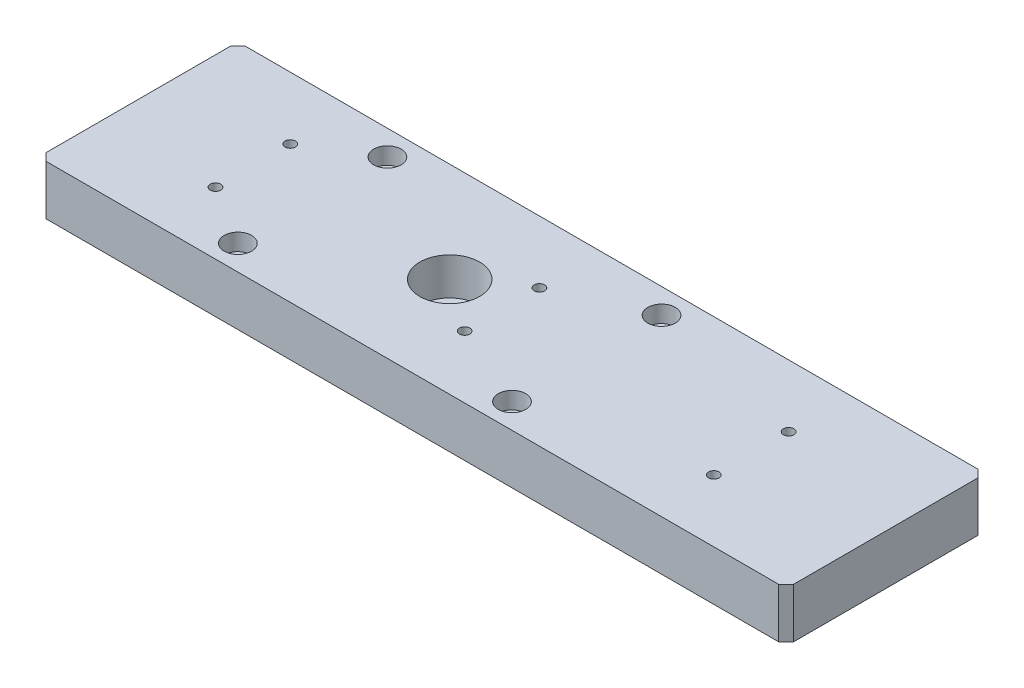
from build123d import *

# Parameters (mm, degrees)
SKETCH_1_W                = 300
SKETCH_1_H                = 80
EXTRUDE_1_DEPTH           = 20
CHAMFER_1_SIZE            = 3
HOLE_WIZARD_1_D           = 15.5
HOLE_WIZARD_1_DEPTH       = 25
HOLE_WIZARD_1_CBORE_D     = 24
HOLE_WIZARD_1_CBORE_DEPTH = 15
HOLE_WIZARD_1_TIP         = 4.656669797
HOLE_WIZARD_0_D           = 6.6
HOLE_WIZARD_0_DEPTH       = 25
HOLE_WIZARD_0_CBORE_D     = 11
HOLE_WIZARD_0_CBORE_DEPTH = 6.8
HOLE_WIZARD_0_TIP         = 1.982840043
SKETCH_6_R                = 10
SKETCH_6_R_2              = 8.1
CUT_EXTRUDE_1_DEPTH       = 2
HOLE_WIZARD_M5_1_D        = 4.2
HOLE_WIZARD_M5_2_D        = 4.2
HOLE_WIZARD_M5_2_DEPTH    = 12.4
HOLE_WIZARD_M5_2_TIP      = 1.2618073


with BuildPart() as part:
    # 草图1 → 凸台-拉伸1 (new body)
    with BuildSketch(Plane(origin=(0, 0, 0), x_dir=(1, 0, 0), z_dir=(0, 1, 0))):
        Rectangle(SKETCH_1_W, SKETCH_1_H)
    extrude(amount=EXTRUDE_1_DEPTH)

    # 倒角1
    chamfer_1_edges = [part.edges().sort_by_distance(p)[0] for p in [
        (150, 10, 40),
        (-150, 10, 40),
        (-150, 10, -40),
        (150, 10, -40),
    ]]
    chamfer(chamfer_1_edges, length=CHAMFER_1_SIZE)

    # 打孔尺寸(%根据)内六角圆柱头螺钉的类型1
    with Locations(Plane(origin=(0, 20, 0), x_dir=(1, 0, 0), z_dir=(0, 1, 0))):
        with Locations((-25, 0)):
            CounterBoreHole(HOLE_WIZARD_1_D / 2, HOLE_WIZARD_1_CBORE_D / 2, HOLE_WIZARD_1_CBORE_DEPTH, depth=HOLE_WIZARD_1_DEPTH)
            with Locations((0, 0, -(HOLE_WIZARD_1_DEPTH + HOLE_WIZARD_1_TIP / 2))):  # 118° drill point
                Cone(0, HOLE_WIZARD_1_D / 2, HOLE_WIZARD_1_TIP, mode=Mode.SUBTRACT)

    # 打孔尺寸(%根据)内六角圆柱头螺钉的类型0
    with Locations(Plane(origin=(0, 20, 0), x_dir=(1, 0, 0), z_dir=(0, 1, 0))):
        with Locations((30, 30), (-80, 30), (30, -30), (-80, -30)):
            CounterBoreHole(HOLE_WIZARD_0_D / 2, HOLE_WIZARD_0_CBORE_D / 2, HOLE_WIZARD_0_CBORE_DEPTH, depth=HOLE_WIZARD_0_DEPTH)
            with Locations((0, 0, -(HOLE_WIZARD_0_DEPTH + HOLE_WIZARD_0_TIP / 2))):  # 118° drill point
                Cone(0, HOLE_WIZARD_0_D / 2, HOLE_WIZARD_0_TIP, mode=Mode.SUBTRACT)

    # 草图6 → 切除-拉伸1 (cut)
    with BuildSketch(Plane.XZ):
        with Locations(Location((-25, 0, 0), (0, 0, 270))):
            Circle(SKETCH_6_R)
        with Locations(Location((30, -30, 0), (0, 0, 270))):
            Circle(SKETCH_6_R_2)
        with Locations(Location((-80, -30, 0), (0, 0, 270))):
            Circle(SKETCH_6_R_2)
        with Locations(Location((30, 30, 0), (0, 0, 270))):
            Circle(SKETCH_6_R_2)
        with Locations(Location((-80, 30, 0), (0, 0, 270))):
            Circle(SKETCH_6_R_2)
    extrude(amount=-CUT_EXTRUDE_1_DEPTH, mode=Mode.SUBTRACT)

    # M5 螺纹孔1 (through all)
    with Locations(Plane(origin=(0, 0, 0), x_dir=(-1, 0, 0), z_dir=(0, -1, 0))):
        with Locations((-96, -15), (-96, 15), (4, -15), (4, 15), (104, -15), (104, 15)):
            Hole(HOLE_WIZARD_M5_1_D / 2)

    # M5 螺纹孔2
    with Locations(Plane(origin=(0, 0, -40), x_dir=(-1, 0, 0), z_dir=(0, 0, -1))):
        with Locations((-142, 10), (-130, 10)):
            Hole(HOLE_WIZARD_M5_2_D / 2, depth=HOLE_WIZARD_M5_2_DEPTH)
            with Locations((0, 0, -(HOLE_WIZARD_M5_2_DEPTH + HOLE_WIZARD_M5_2_TIP / 2))):  # 118° drill point
                Cone(0, HOLE_WIZARD_M5_2_D / 2, HOLE_WIZARD_M5_2_TIP, mode=Mode.SUBTRACT)


solid = part.part
